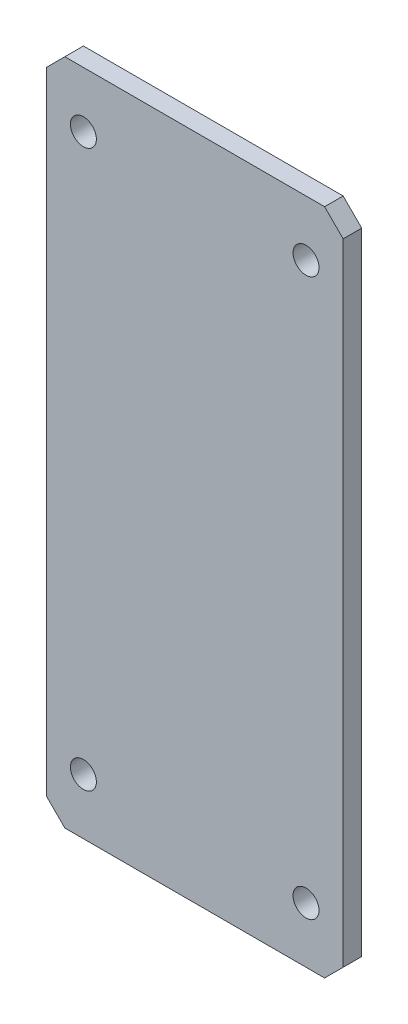
SolidWorks part; units mm, degrees
material "1023 碳钢板 (SS)"
ref_plane "前视基准面" through (0, 0, 0) normal (0, 0, 1) x (1, 0, 0)
ref_plane "上视基准面" through (0, 0, 0) normal (0, 1, 0) x (1, 0, 0)
ref_plane "右视基准面" through (0, 0, 0) normal (1, 0, 0) x (0, 0, -1)
sketch "草图1" plane through (0, 0, 0) normal (0, 0, 1) x (1, 0, 0)
  line L1 (-40, 90) -> (40, 90)
  line L2 (-40, 90) -> (-40, -90)
  line L3 (-40, -90) -> (40, -90)
  line L4 (40, 90) -> (40, -90)
  line L5 (-40, 90) -> (40, -90) construction
  line L6 (-40, -90) -> (40, 90) construction
  point P0 (0, 0)
  dimension "D1" = 180
  dimension "D2" = 80
extrude "凸台-拉伸1" add sketch "草图1" along normal blind 5
chamfer "倒角1" distance 5 angle 45 4 edges at (-40, -90, 2.5) (40, -90, 2.5) (40, 90, 2.5) (-40, 90, 2.5)
sketch "草图2" plane through (0, 0, 5) normal (0, 0, 1) x (1, 0, 0)
  circle A0 centre (-30, 75) radius 3.5
  circle A1 centre (30, 75) radius 3.5
  circle A2 centre (-30, -75) radius 3.5
  circle A3 centre (30, -75) radius 3.5
  point P8 (0, 0)
  point P9 (0, 0)
  point P10 (0, 0)
  point P11 (0, 0)
  dimension "D5" = 7
  dimension "D1" = 60
  dimension "D2" = 150
  dimension "D3" = 30
  dimension "D4" = 75
extrude "切除-拉伸1" cut sketch "草图2" against normal blind 5
